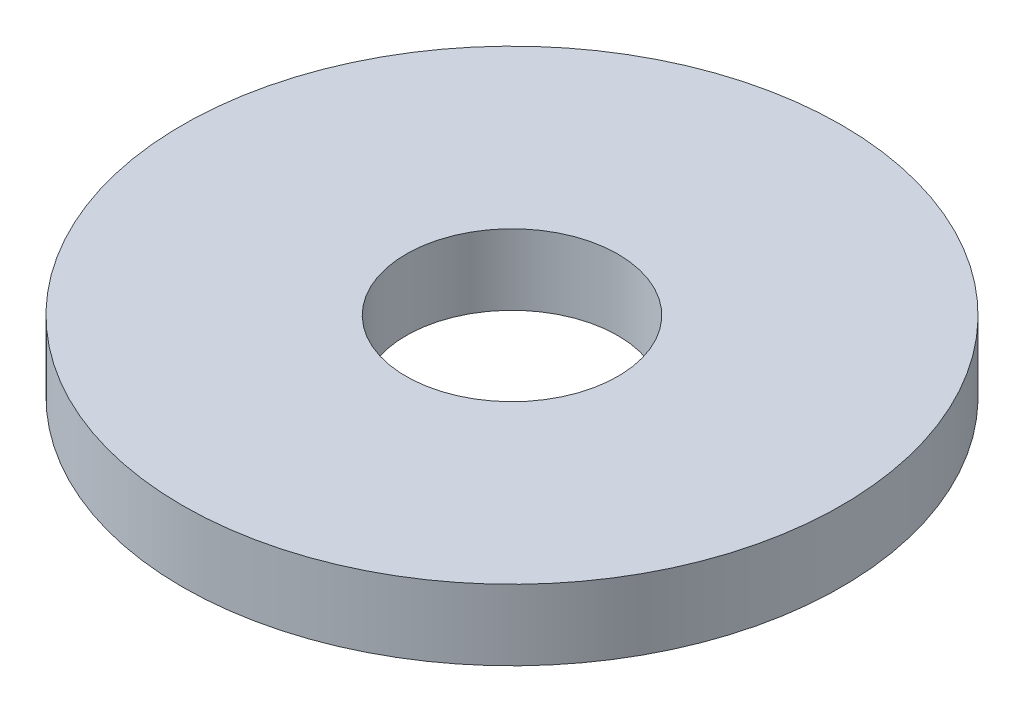
from build123d import *

# Parameters (mm, degrees)
SKETCH_1_W = 9.5
SKETCH_1_H = 3


with BuildPart() as part:
    # 草图1 → Revolve 468 (revolve)
    with BuildSketch(Plane.XY, mode=Mode.PRIVATE) as revolve_468_sk:
        with Locations((-9.25, 10.144507042)):
            Rectangle(SKETCH_1_W, SKETCH_1_H)
    revolve(revolve_468_sk.sketch.rotate(Axis((0, 0, 0), (0, 1, 0)), 270), axis=Axis((0, 0, 0), (0, 1, 0)))


solid = part.part
